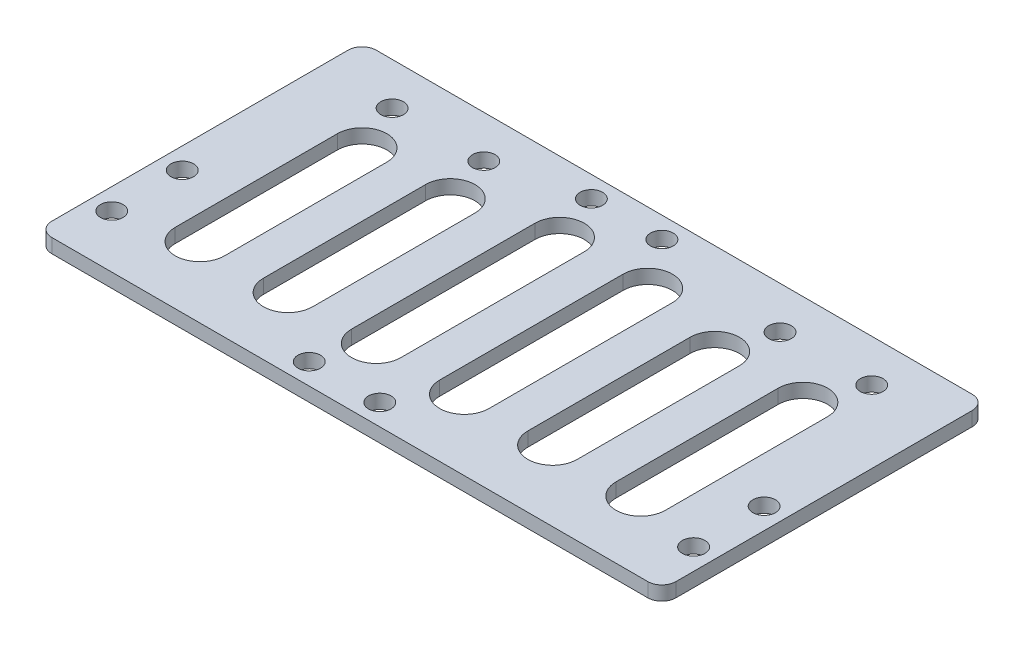
from build123d import *

# Parameters (mm, degrees)
SKETCH_1_W          = 88.5
SKETCH_1_H          = 46
SKETCH_1_R          = 1.6
EXTRUDE_1_DEPTH     = 2
CUT_EXTRUDE_1_DEPTH = 50.910544978
FILLET_1_R          = 2


with BuildPart() as part:
    # 草图1 → 凸台-拉伸1 (new body)
    with BuildSketch(Plane(origin=(0, 0, 0), x_dir=(1, 0, 0), z_dir=(0, 1, 0))):
        Rectangle(SKETCH_1_W, SKETCH_1_H)
        with Locations(Location((-41.25, -5.5, 0), (0, 0, 270))):
            Circle(SKETCH_1_R, mode=Mode.SUBTRACT)
        with Locations(Location((-41.25, -15.5, 0), (0, 0, 270))):
            Circle(SKETCH_1_R, mode=Mode.SUBTRACT)
        with Locations(Location((41.25, -15.5, 0), (0, 0, 90))):
            Circle(SKETCH_1_R, mode=Mode.SUBTRACT)
        with Locations(Location((41.25, -5.5, 0), (0, 0, 90))):
            Circle(SKETCH_1_R, mode=Mode.SUBTRACT)
        with Locations(Location((-8.75, -20, 0), (0, 0, 270))):
            Circle(SKETCH_1_R, mode=Mode.SUBTRACT)
        with Locations(Location((1.25, -20, 0), (0, 0, 270))):
            Circle(SKETCH_1_R, mode=Mode.SUBTRACT)
        with Locations(Location((-34, 17, 0), (0, 0, 270))):
            Circle(SKETCH_1_R, mode=Mode.SUBTRACT)
        with Locations(Location((-21, 17, 0), (0, 0, 270))):
            Circle(SKETCH_1_R, mode=Mode.SUBTRACT)
        with Locations(Location((21, 17, 0), (0, 0, 270))):
            Circle(SKETCH_1_R, mode=Mode.SUBTRACT)
        with Locations(Location((34, 17, 0), (0, 0, 270))):
            Circle(SKETCH_1_R, mode=Mode.SUBTRACT)
        with Locations(Location((1.25, 20, 0), (0, 0, 90))):
            Circle(SKETCH_1_R, mode=Mode.SUBTRACT)
        with Locations(Location((-8.75, 20, 0), (0, 0, 90))):
            Circle(SKETCH_1_R, mode=Mode.SUBTRACT)
    extrude(amount=EXTRUDE_1_DEPTH)

    # 草图2 → 切除-拉伸1 (cut, through all)
    with BuildSketch(Plane(origin=(0, 2, 0), x_dir=(1, 0, 0), z_dir=(0, 1, 0))):
        with BuildLine():
            Line((-27.75, 10), (-27.75, -13))
            ThreePointArc((-27.75, -13), (-31.25, -16.5), (-34.75, -13))
            Line((-34.75, -13), (-34.75, 10))
            ThreePointArc((-34.75, 10), (-31.25, 13.5), (-27.75, 10))
        make_face()
        with BuildLine():
            Line((-15.25, 10), (-15.25, -13))
            ThreePointArc((-15.25, -13), (-18.75, -16.5), (-22.25, -13))
            Line((-22.25, -13), (-22.25, 10))
            ThreePointArc((-22.25, 10), (-18.75, 13.5), (-15.25, 10))
        make_face()
        with BuildLine():
            Line((-2.75, 13), (-2.75, -13))
            ThreePointArc((-2.75, -13), (-6.25, -16.5), (-9.75, -13))
            Line((-9.75, -13), (-9.75, 13))
            ThreePointArc((-9.75, 13), (-6.25, 16.5), (-2.75, 13))
        make_face()
        with BuildLine():
            Line((9.75, 13), (9.75, -13))
            ThreePointArc((9.75, -13), (6.25, -16.5), (2.75, -13))
            Line((2.75, -13), (2.75, 13))
            ThreePointArc((2.75, 13), (6.25, 16.5), (9.75, 13))
        make_face()
        with BuildLine():
            Line((22.25, 10), (22.25, -13))
            ThreePointArc((22.25, -13), (18.75, -16.5), (15.25, -13))
            Line((15.25, -13), (15.25, 10))
            ThreePointArc((15.25, 10), (18.75, 13.5), (22.25, 10))
        make_face()
        with BuildLine():
            Line((34.75, 10), (34.75, -13))
            ThreePointArc((34.75, -13), (31.25, -16.5), (27.75, -13))
            Line((27.75, -13), (27.75, 10))
            ThreePointArc((27.75, 10), (31.25, 13.5), (34.75, 10))
        make_face()
    extrude(amount=-CUT_EXTRUDE_1_DEPTH, mode=Mode.SUBTRACT)

    # 圆角1
    fillet_1_edges = [part.edges().sort_by_distance(p)[0] for p in [
        (44.25, 1, 23),
        (-44.25, 1, 23),
        (-44.25, 1, -23),
        (44.25, 1, -23),
    ]]
    fillet(fillet_1_edges, radius=FILLET_1_R)


solid = part.part
